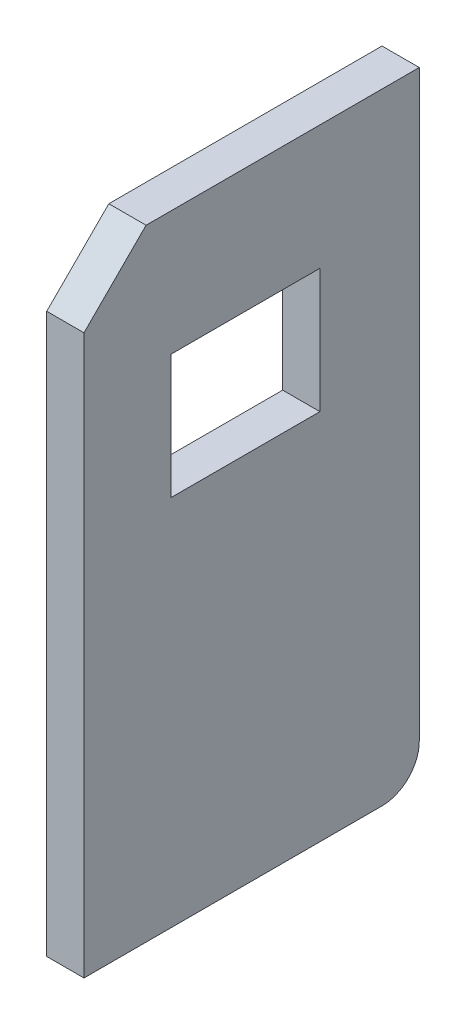
SolidWorks part; units mm, degrees
material "Q235A"
ref_plane "前视基准面" through (0, 0, 0) normal (0, 0, 1) x (1, 0, 0)
ref_plane "上视基准面" through (0, 0, 0) normal (0, 1, 0) x (1, 0, 0)
ref_plane "右视基准面" through (0, 0, 0) normal (1, 0, 0) x (0, 0, -1)
sketch "草图1" plane through (0, 0, 0) normal (1, 0, 0) x (0, 0, -1)
  line L0 (-22, 50) -> (-27, 45)
  line L1 (-27, 45) -> (-27, 0)
  line L2 (-27, 0) -> (0, 0)
  line L3 (0, 0) -> (0, 50)
  line L4 (0, 50) -> (-22, 50)
  dimension "D1" = 5
  dimension "D2" = 5
  dimension "D3" = 27
  dimension "D4" = 50
extrude "凸台-拉伸1" add sketch "草图1" along normal blind 3
fillet "圆角1" radius 3 1 edges at (1.5, 0, 0)
sketch "草图2" plane through (3, 0, 0) normal (1, 0, 0) x (0, 0, -1)
  line L1 (-20, 30) -> (-8, 30)
  line L2 (-20, 30) -> (-20, 40)
  line L3 (-20, 40) -> (-8, 40)
  line L4 (-8, 30) -> (-8, 40)
  line L5 (-27, 0) -> (-3, 0) construction
  line L6 (0, 3) -> (0, 50) construction
  dimension "D1" = 8
  dimension "D2" = 12
  dimension "D3" = 30
  dimension "D4" = 10
extrude "切除-拉伸1" cut sketch "草图2" against normal through all
equation "\"Hd\"= \"D1@凸台-拉伸1\""
